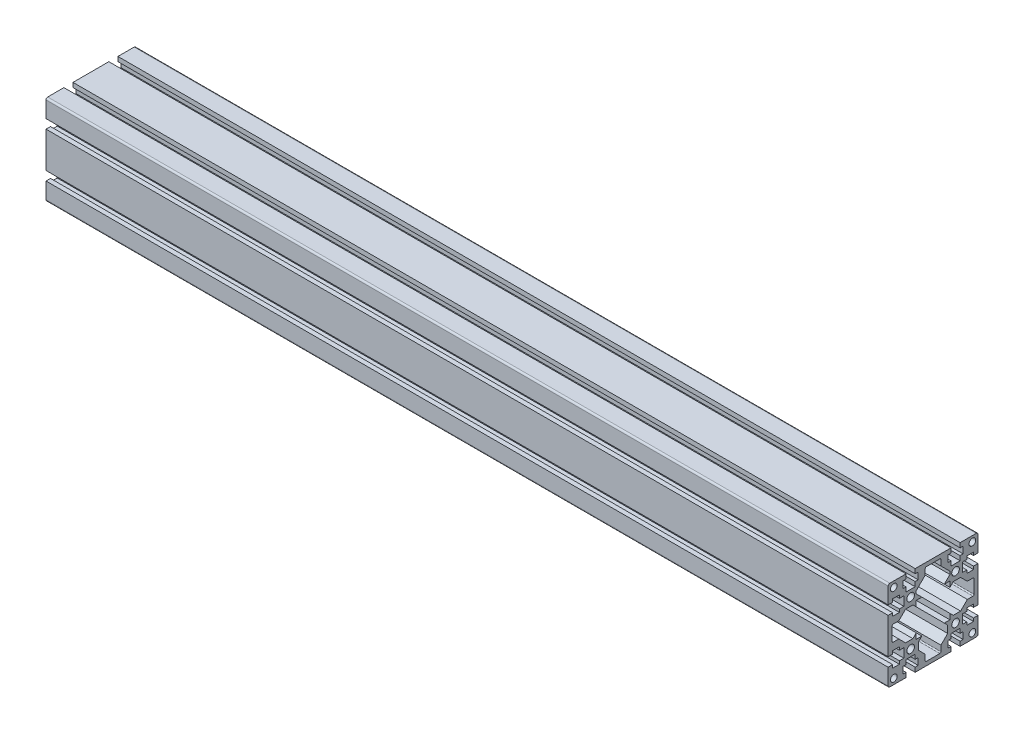
from build123d import *

# Parameters (mm, degrees)
SKETCH1_R                                 = 3.4
SKETCH1_R_2                               = 3
ALUMINIUM_PROFILE_80_X_80G_X_R1_5_1_DEPTH = 750
SKETCH10_R                                = 3
CUT_EXTRUDE1_DEPTH                        = 753.130307859


with BuildPart() as part:
    # Sketch1 → Aluminium profile 80 X 80G X R1.5(1) (new body)
    with BuildSketch(Plane.YZ.offset(-530.344827586)):
        with BuildLine():
            Line((-24.05, 40), (-24.05, 36))
            Line((-24.05, 36), (-26.75, 36))
            Line((-26.75, 36), (-26.75, 30))
            Line((-26.75, 30), (-24.05, 30))
            Line((-24.05, 30), (-24.05, 26))
            Line((-24.05, 26), (-15.95, 26))
            Line((-15.95, 26), (-15.95, 30))
            Line((-15.95, 30), (-13.25, 30))
            Line((-13.25, 30), (-13.25, 36))
            Line((-13.25, 36), (-15.95, 36))
            Line((-15.95, 36), (-15.95, 40))
            Line((-15.95, 40), (15.95, 40))
            Line((15.95, 40), (15.95, 36))
            Line((15.95, 36), (13.25, 36))
            Line((13.25, 36), (13.25, 30))
            Line((13.25, 30), (15.95, 30))
            Line((15.95, 30), (15.95, 26))
            Line((15.95, 26), (24.05, 26))
            Line((24.05, 26), (24.05, 30))
            Line((24.05, 30), (26.75, 30))
            Line((26.75, 30), (26.75, 36))
            Line((26.75, 36), (24.05, 36))
            Line((24.05, 36), (24.05, 40))
            Line((24.05, 40), (38.5, 40))
            ThreePointArc((38.5, 40), (39.560660172, 39.560660172), (40, 38.5))
            Line((40, 38.5), (40, 24.05))
            Line((40, 24.05), (36, 24.05))
            Line((36, 24.05), (36, 26.75))
            Line((36, 26.75), (30, 26.75))
            Line((30, 26.75), (30, 24.05))
            Line((30, 24.05), (26, 24.05))
            Line((26, 24.05), (26, 15.95))
            Line((26, 15.95), (30, 15.95))
            Line((30, 15.95), (30, 13.25))
            Line((30, 13.25), (36, 13.25))
            Line((36, 13.25), (36, 15.95))
            Line((36, 15.95), (40, 15.95))
            Line((40, 15.95), (40, -15.95))
            Line((40, -15.95), (36, -15.95))
            Line((36, -15.95), (36, -13.25))
            Line((36, -13.25), (30, -13.25))
            Line((30, -13.25), (30, -15.95))
            Line((30, -15.95), (26, -15.95))
            Line((26, -15.95), (26, -24.05))
            Line((26, -24.05), (30, -24.05))
            Line((30, -24.05), (30, -26.75))
            Line((30, -26.75), (36, -26.75))
            Line((36, -26.75), (36, -24.05))
            Line((36, -24.05), (40, -24.05))
            Line((40, -24.05), (40, -38.5))
            ThreePointArc((40, -38.5), (39.560660172, -39.560660172), (38.5, -40))
            Line((38.5, -40), (24.05, -40))
            Line((24.05, -40), (24.05, -36))
            Line((24.05, -36), (26.75, -36))
            Line((26.75, -36), (26.75, -30))
            Line((26.75, -30), (24.05, -30))
            Line((24.05, -30), (24.05, -26))
            Line((24.05, -26), (15.95, -26))
            Line((15.95, -26), (15.95, -30))
            Line((15.95, -30), (13.25, -30))
            Line((13.25, -30), (13.25, -36))
            Line((13.25, -36), (15.95, -36))
            Line((15.95, -36), (15.95, -40))
            Line((15.95, -40), (-15.95, -40))
            Line((-15.95, -40), (-15.95, -36))
            Line((-15.95, -36), (-13.25, -36))
            Line((-13.25, -36), (-13.25, -30))
            Line((-13.25, -30), (-15.95, -30))
            Line((-15.95, -30), (-15.95, -26))
            Line((-15.95, -26), (-24.05, -26))
            Line((-24.05, -26), (-24.05, -30))
            Line((-24.05, -30), (-26.75, -30))
            Line((-26.75, -30), (-26.75, -36))
            Line((-26.75, -36), (-24.05, -36))
            Line((-24.05, -36), (-24.05, -40))
            Line((-24.05, -40), (-38.5, -40))
            ThreePointArc((-38.5, -40), (-39.560660172, -39.560660172), (-40, -38.5))
            Line((-40, -38.5), (-40, -24.05))
            Line((-40, -24.05), (-36, -24.05))
            Line((-36, -24.05), (-36, -26.75))
            Line((-36, -26.75), (-30, -26.75))
            Line((-30, -26.75), (-30, -24.05))
            Line((-30, -24.05), (-26, -24.05))
            Line((-26, -24.05), (-26, -15.95))
            Line((-26, -15.95), (-30, -15.95))
            Line((-30, -15.95), (-30, -13.25))
            Line((-30, -13.25), (-36, -13.25))
            Line((-36, -13.25), (-36, -15.95))
            Line((-36, -15.95), (-40, -15.95))
            Line((-40, -15.95), (-40, 15.95))
            Line((-40, 15.95), (-36, 15.95))
            Line((-36, 15.95), (-36, 13.25))
            Line((-36, 13.25), (-30, 13.25))
            Line((-30, 13.25), (-30, 15.95))
            Line((-30, 15.95), (-26, 15.95))
            Line((-26, 15.95), (-26, 24.05))
            Line((-26, 24.05), (-30, 24.05))
            Line((-30, 24.05), (-30, 26.75))
            Line((-30, 26.75), (-36, 26.75))
            Line((-36, 26.75), (-36, 24.05))
            Line((-36, 24.05), (-40, 24.05))
            Line((-40, 24.05), (-40, 38.5))
            ThreePointArc((-40, 38.5), (-39.560660172, 39.560660172), (-38.5, 40))
            Line((-38.5, 40), (-24.05, 40))
        make_face()
        with Locations((-20, 20)):
            Circle(SKETCH1_R, mode=Mode.SUBTRACT)
        with Locations((20, 20)):
            Circle(SKETCH1_R, mode=Mode.SUBTRACT)
        with Locations((20, -20)):
            Circle(SKETCH1_R, mode=Mode.SUBTRACT)
        with Locations((-20, -20)):
            Circle(SKETCH1_R, mode=Mode.SUBTRACT)
        with Locations((-35, 35)):
            Circle(SKETCH1_R_2, mode=Mode.SUBTRACT)
        with Locations((35, 35)):
            Circle(SKETCH1_R_2, mode=Mode.SUBTRACT)
        with Locations((35, -35)):
            Circle(SKETCH1_R_2, mode=Mode.SUBTRACT)
        with BuildLine():
            Line((-13, 18), (-10, 15))
            Line((-10, 15), (-15, 15))
            Line((-15, 15), (-15, 10))
            Line((-15, 10), (-18, 13))
            Line((-18, 13), (-24.5, 13))
            Line((-24.5, 13), (-30.5, 7))
            Line((-30.5, 7), (-35.5, 7))
            ThreePointArc((-35.5, 7), (-36.207106781, 6.707106781), (-36.5, 6))
            Line((-36.5, 6), (-36.5, -6))
            ThreePointArc((-36.5, -6), (-36.207106781, -6.707106781), (-35.5, -7))
            Line((-35.5, -7), (-30.5, -7))
            Line((-30.5, -7), (-24.5, -13))
            Line((-24.5, -13), (-18, -13))
            Line((-18, -13), (-15, -10))
            Line((-15, -10), (-15, -15))
            Line((-15, -15), (-10, -15))
            Line((-10, -15), (-13, -18))
            Line((-13, -18), (-13, -24.5))
            Line((-13, -24.5), (-7, -30.5))
            Line((-7, -30.5), (-7, -35.5))
            ThreePointArc((-7, -35.5), (-6.707106781, -36.207106781), (-6, -36.5))
            Line((-6, -36.5), (6, -36.5))
            ThreePointArc((6, -36.5), (6.707106781, -36.207106781), (7, -35.5))
            Line((7, -35.5), (7, -30.5))
            Line((7, -30.5), (13, -24.5))
            Line((13, -24.5), (13, -18))
            Line((13, -18), (10, -15))
            Line((10, -15), (15, -15))
            Line((15, -15), (15, -10))
            Line((15, -10), (20, -15))
            Line((20, -15), (22.5, -15))
            Line((22.5, -15), (30.5, -7))
            Line((30.5, -7), (35.5, -7))
            ThreePointArc((35.5, -7), (36.207106781, -6.707106781), (36.5, -6))
            Line((36.5, -6), (36.5, 6))
            ThreePointArc((36.5, 6), (36.207106781, 6.707106781), (35.5, 7))
            Line((35.5, 7), (30.5, 7))
            Line((30.5, 7), (22.5, 15))
            Line((22.5, 15), (20, 15))
            Line((20, 15), (15, 10))
            Line((15, 10), (15, 15))
            Line((15, 15), (10, 15))
            Line((10, 15), (13, 18))
            Line((13, 18), (13, 24.5))
            Line((13, 24.5), (7, 30.5))
            Line((7, 30.5), (7, 35.5))
            ThreePointArc((7, 35.5), (6.707106781, 36.207106781), (6, 36.5))
            Line((6, 36.5), (-6, 36.5))
            ThreePointArc((-6, 36.5), (-6.707106781, 36.207106781), (-7, 35.5))
            Line((-7, 35.5), (-7, 30.5))
            Line((-7, 30.5), (-13, 24.5))
            Line((-13, 24.5), (-13, 18))
        make_face(mode=Mode.SUBTRACT)
    extrude(amount=ALUMINIUM_PROFILE_80_X_80G_X_R1_5_1_DEPTH)

    # Sketch10 → Cut-Extrude1 (cut, through all)
    with BuildSketch(Plane(origin=(219.655172414, 0, 0), x_dir=(0, 0, -1), z_dir=(1, 0, 0))):
        with Locations((35, -35)):
            Circle(SKETCH10_R)
    extrude(amount=-CUT_EXTRUDE1_DEPTH, mode=Mode.SUBTRACT)


solid = part.part
